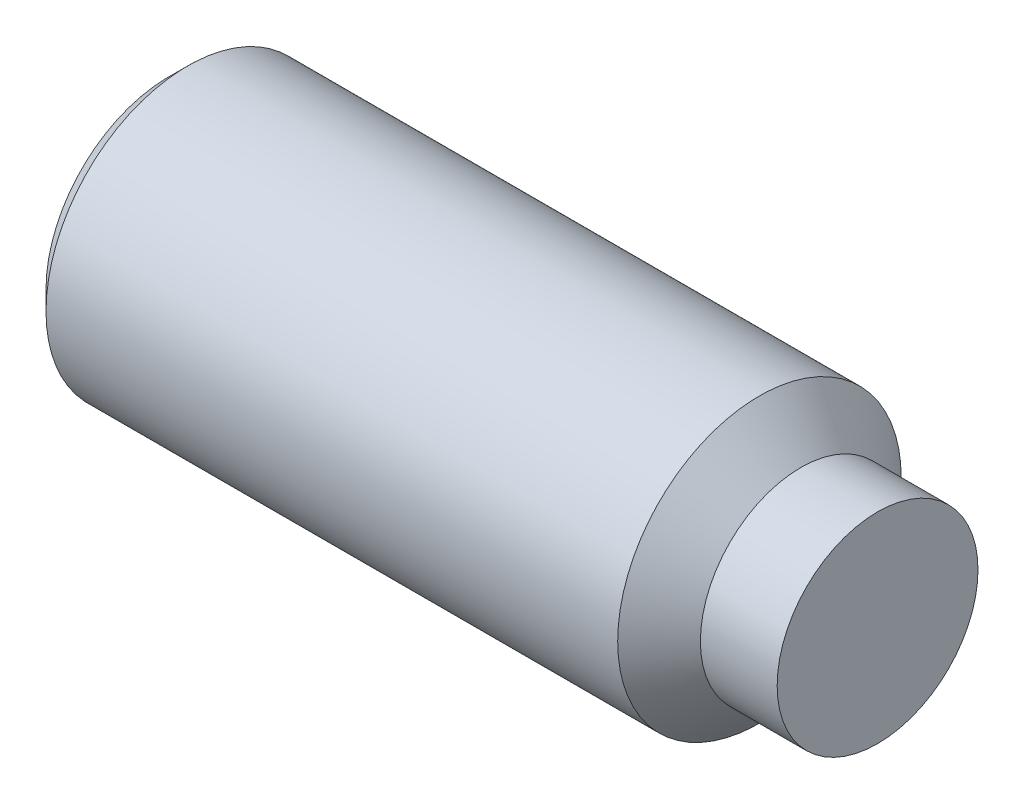
SolidWorks part; units mm, degrees
revolve "基体-旋转" add sketch "草图1" angle 360 about L7
sketch "草图1" plane through (0, 0, 0) normal (0, 0, 1) x (1, 0, 0)
  line L0 (0, 0) -> (30, 0)
  line L1 (30, 0) -> (30, 4.25)
  line L2 (30, 4.25) -> (26.75, 4.25)
  line L3 (26.75, 4.25) -> (25, 6)
  line L4 (25, 6) -> (0.804, 6)
  line L5 (0.804, 6) -> (0, 5.196)
  line L6 (0, 5.196) -> (0, 0)
  line L7 (-0.6655, 0) -> (5.3015, 0) construction
cosmetic thread "装饰螺纹线1" parameters "D1"=25, "df"=10.392
material "45H级"
ref_plane "前视" through (0, 0, 0) normal (0, 0, 1) x (1, 0, 0)
ref_plane "上视" through (0, 0, 0) normal (0, 1, 0) x (1, 0, 0)
ref_plane "右视" through (0, 0, 0) normal (1, 0, 0) x (0, 0, -1)
sketch "尺寸草图" plane through (0, 0, 0) normal (0, 0, 1) x (1, 0, 0)
  line L0 (0, 0) -> (30, 0)
  point P3 (10.392, 0)
  point P4 (4.8, 0)
  point P5 (12, 0)
  point P6 (28.25, 0)
  point P7 (21.5, 0)
  point P8 (23.14, 0)
  point P9 (26.75, 0)
sketch "草图2" plane through (0, 0, 0) normal (-1, 0, 0) x (0, 0, 1)
  line L1 (3.43, 0) -> (1.715, 2.9705)
  line L2 (1.715, 2.9705) -> (-1.715, 2.9705)
  line L3 (-1.715, 2.9705) -> (-3.43, 0)
  line L4 (-3.43, 0) -> (-1.715, -2.9705)
  line L5 (-1.715, -2.9705) -> (1.715, -2.9705)
  line L6 (1.715, -2.9705) -> (3.43, 0)
  circle A0 centre (0, 0) radius 2.9705 construction
extrude "切除-拉伸1" cut sketch "草图2" against normal blind 4.8
sketch "草图3" plane through (0, 0, 0) normal (0, 0, 1) x (1, 0, 0)
  line L0 (-0.2621, 0) -> (1.1933, 0) construction
  line L1 (-0.6655, 0) -> (5.3015, 0) construction
  line L2 (4.8, 2.9705) -> (6.515, 0)
  line L3 (6.515, 0) -> (4.8, 0)
  line L4 (4.8, 0) -> (4.8, 2.9705)
  dimension "D1" = 60
revolve "切除-旋转1" cut sketch "草图3" angle 360 about L0
sketch "草图4" plane through (0, 0, 0) normal (0, 0, 1) x (1, 0, 0)
  line L0 (0.804, 6) -> (2.554, 6)
  line L1 (2.554, 6) -> (1.6695, 4.4845)
  line L2 (1.6695, 4.4845) -> (0.804, 6)
  line L3 (25, 6) -> (0.804, 6) construction
  line L4 (0.804, 6) -> (0.804, -6) construction
  line L5 (-0.1839, 0) -> (5.1682, 0) construction
  line L6 (-0.6655, 0) -> (5.3015, 0) construction
revolve "切除-旋转2" [suppressed] cut sketch "草图4" angle 360 about L5
pattern_linear "阵列(线性)1" [suppressed] count 14
equation "\"l@草图1\" = \"l@尺寸草图\""
equation "\"d@草图1\" = \"d@尺寸草图\""
equation "\"df@草图1\" = \"df@尺寸草图\""
equation "\"dp@草图1\" = \"dp@尺寸草图\""
equation "\"z@草图1\" = \"z@尺寸草图\""
equation "\"df@装饰螺纹线1\" = \"df@尺寸草图\""
equation "\"e@草图2\" = \"e@尺寸草图\""
equation "\"t@切除-拉伸1\" = \"t@尺寸草图\""
equation "\"P@草图4\" = \"P@尺寸草图\""
equation "\"D1@草图4\" = \"P@尺寸草图\"*0.866"
equation "\"P@阵列(线性)1\" = \"P@尺寸草图\""
equation "\"D1@阵列(线性)1\" = (\"l@尺寸草图\"-\"z@尺寸草图\"-\"d@尺寸草图\"/2+\"dp@尺寸草图\"/2)/\"P@尺寸草图\""
equation "\"D1@装饰螺纹线1\"=\"l@尺寸草图\"-\"z@尺寸草图\"-\"d@尺寸草图\"/2+\"dp@尺寸草图\"/2"
